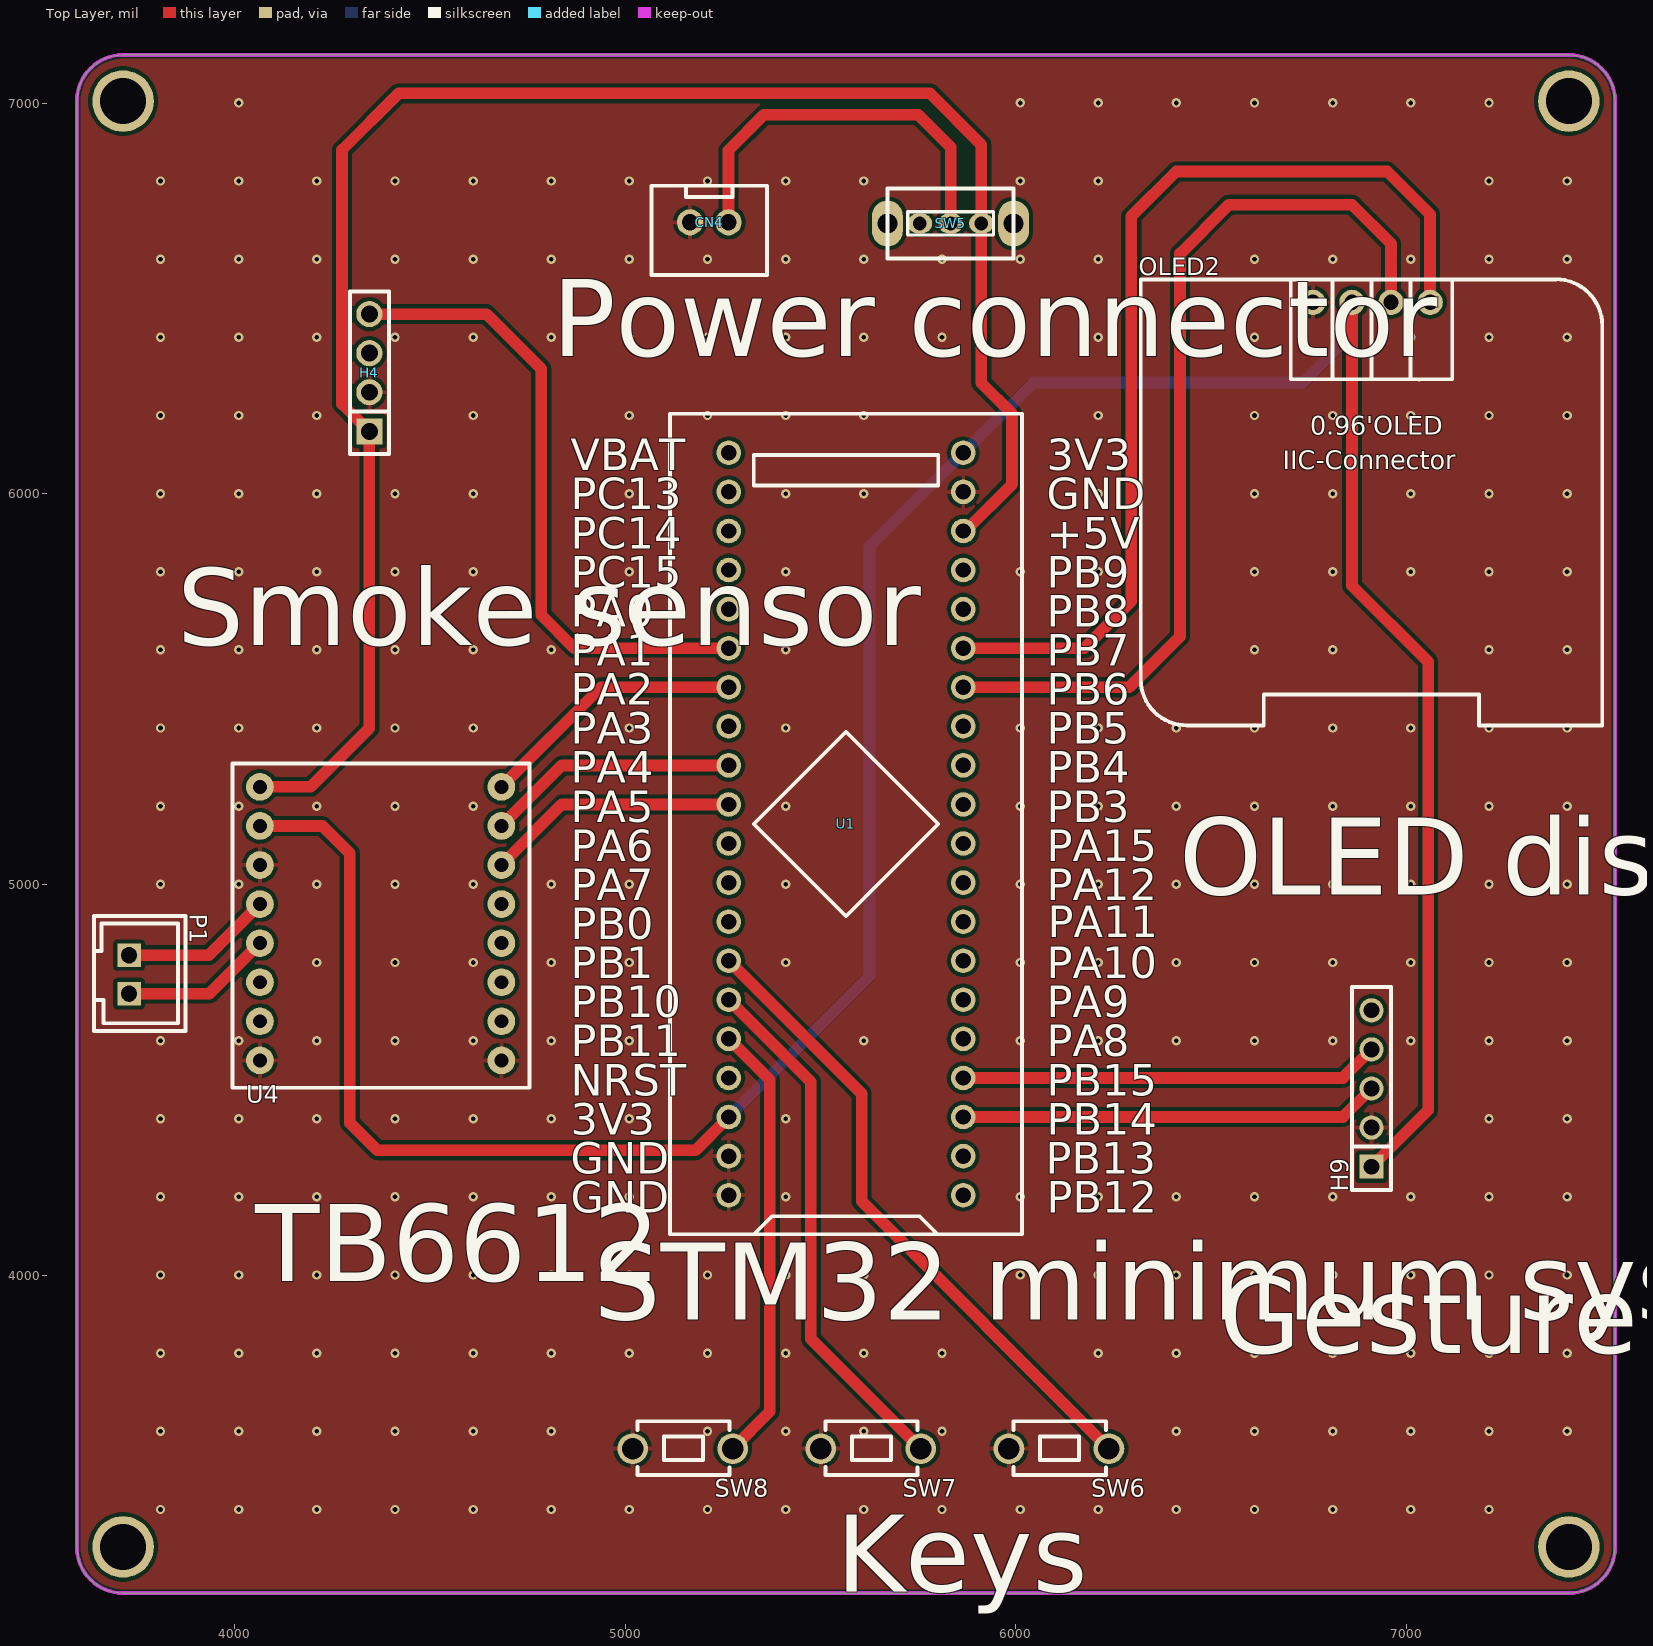
[diagram p0: Top Layer view]
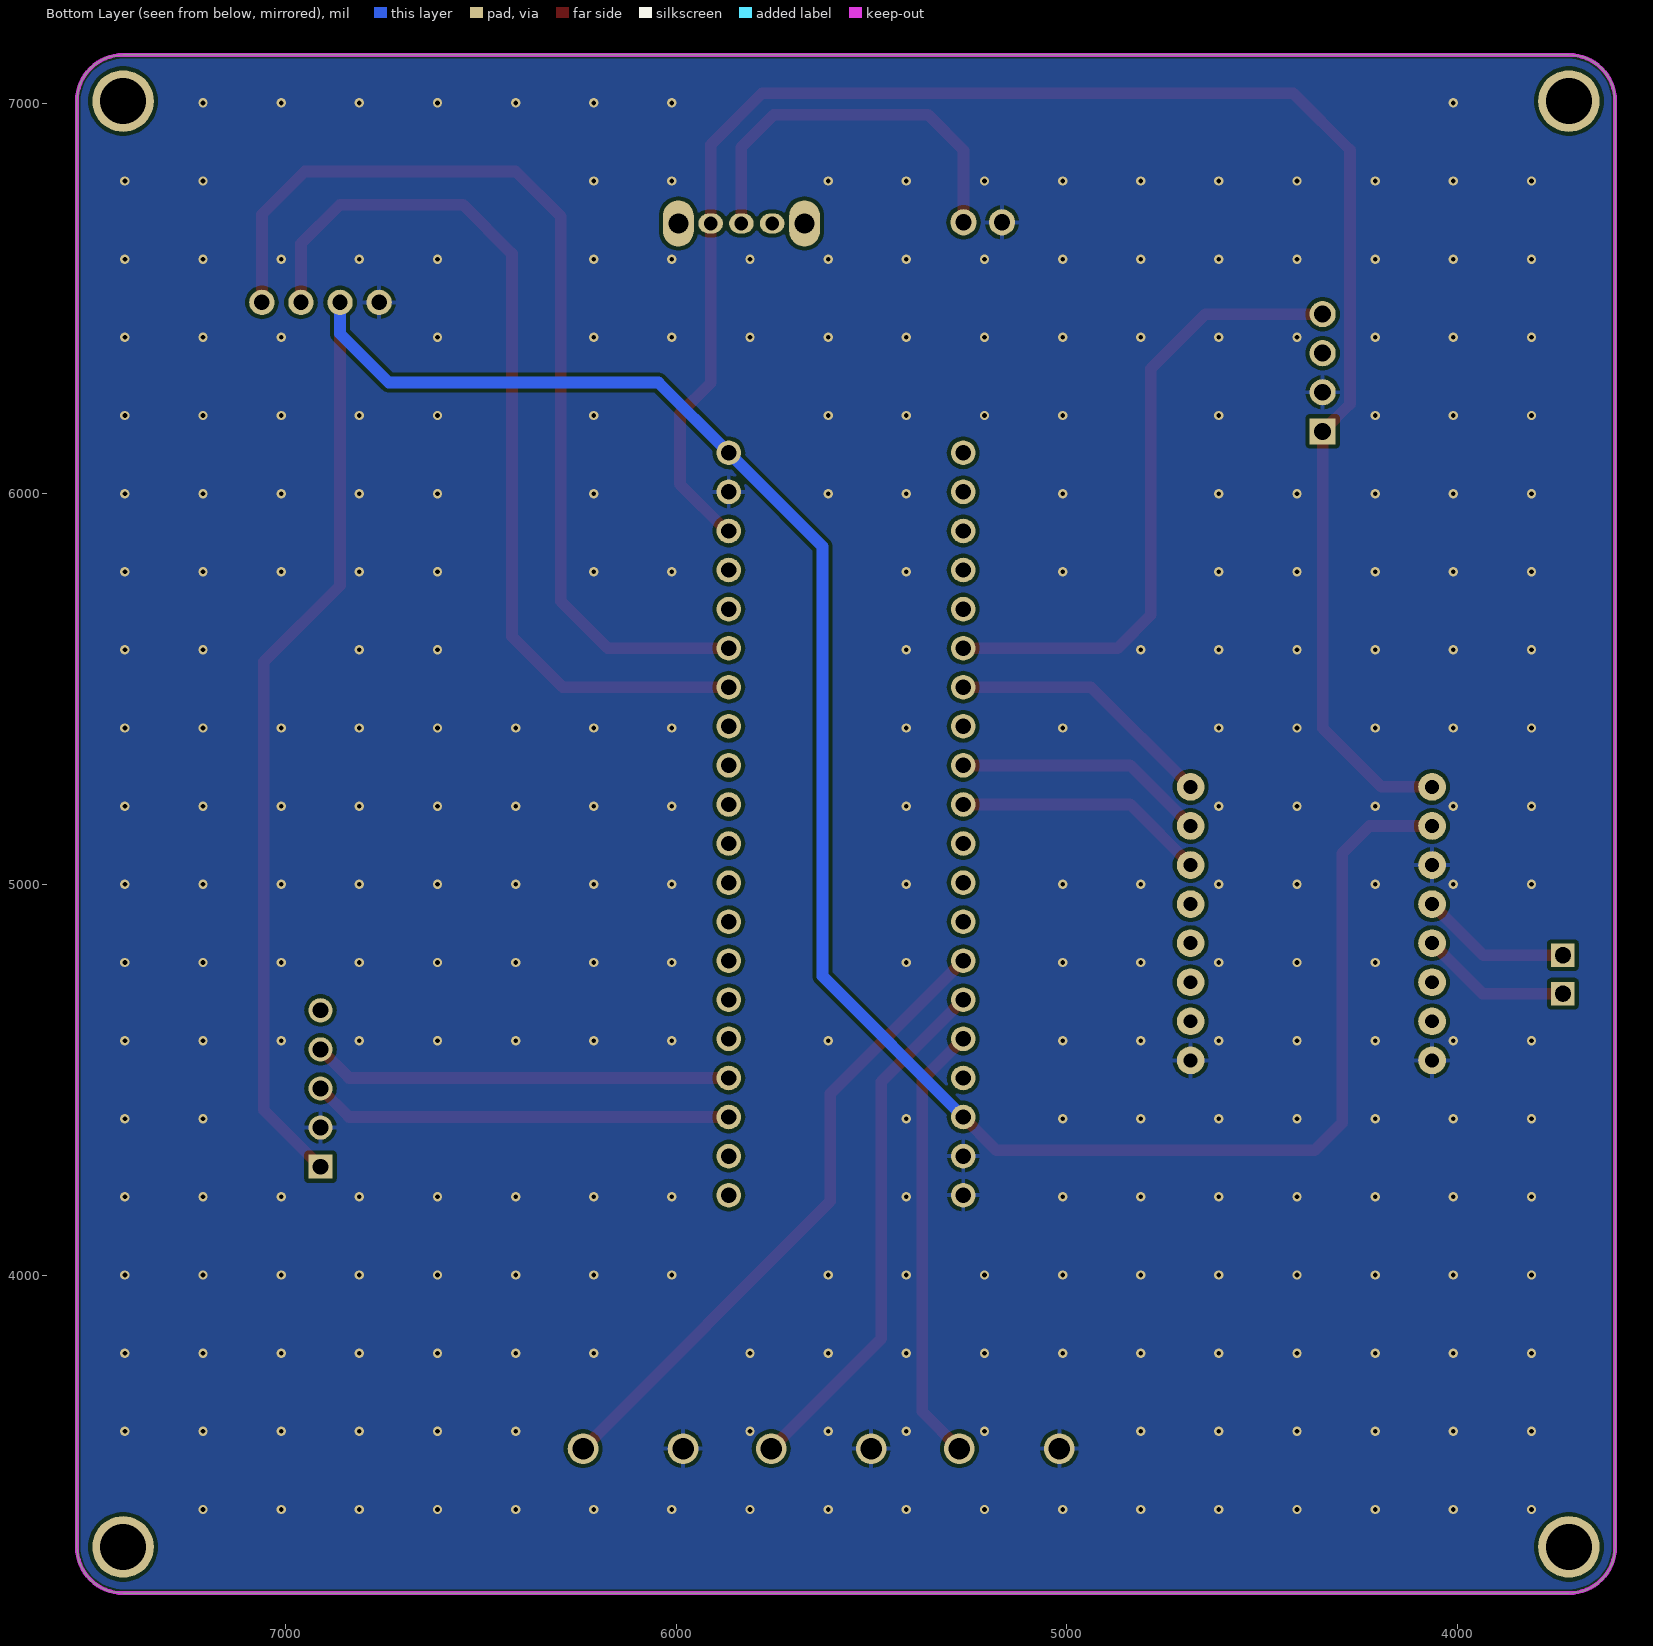
[diagram p1: Bottom Layer view, seen from below]
# Altium PCB MISC89068.pcbdoc
Units mil, origin at the board's own origin, x right, y up, seen from the top; angles counter-clockwise.
Board outline 3937.01 x 3937.01 mil, 2 copper layers (Top Layer, Bottom Layer), stack 62.206 mil thick; 11 components, 40 nets, 88 pads, 281 vias.

## Layer stack, top to bottom
Top Solder Mask Layer: solder mask 0.394, Dk 3.3
Top Layer: signal copper 1.379
Dielectric1: surface 59.449, FR4, Dk 4.5
Bottom Layer: signal copper 1.378
Bottom Solder Mask Layer: solder mask 0.394, Dk 3.3

## Board outline
3714.61,7123.5 ccw(c3714.61,7005.39) 3596.5,7005.39 3596.5,3304.61 ccw(c3714.61,3304.61) 3714.61,3186.5 7415.39,3186.5 ccw(c7415.39,3304.61) 7533.5,3304.61 7533.5,7005.39 ccw(c7415.39,7005.39) 7415.39,7123.5 3714.61,7123.5

## Design rules (kind name [scope] priority, off if disabled: settings)
BoardOutlineClearance copperThickness2oz_1 [All] p2 off: genericclearance=7.99 ignorepadtopadclearanceinfootprint=FALSE except(0: Arc-SplitContinuation Track-SplitContinuation SMDPad-SplitContinuation THPad-SplitContinuation Via-SplitContinuation Fill-SplitContinuation Region-SplitContinuation Poly-SplitContinuation Text-SplitContinuation Hole-SplitContinuation; 5.98: Arc-CutoutEdge Track-CutoutEdge SMDPad-CutoutEdge THPad-CutoutEdge Via-CutoutEdge Text-CutoutEdge; 6.9: Hole-OutlineEdge Hole-CutoutEdge; 10: Poly-OutlineEdge Poly-CutoutEdge; 11.81: Arc-OutlineEdge Track-OutlineEdge SMDPad-OutlineEdge THPad-OutlineEdge Via-OutlineEdge Fill-OutlineEdge Region-OutlineEdge Text-OutlineEdge Fill-CutoutEdge Region-CutoutEdge)
BoardOutlineClearance Plane_innerPlane_1 [All] p4 off: genericclearance=4.02 ignorepadtopadclearanceinfootprint=FALSE except(0: Arc-SplitContinuation Track-SplitContinuation SMDPad-SplitContinuation THPad-SplitContinuation Via-SplitContinuation Fill-SplitContinuation Region-SplitContinuation Poly-SplitContinuation Text-SplitContinuation Hole-SplitContinuation; 5.98: Arc-CutoutEdge Track-CutoutEdge SMDPad-CutoutEdge THPad-CutoutEdge Via-CutoutEdge Text-CutoutEdge; 6.9: Hole-OutlineEdge Hole-CutoutEdge; 10: Poly-OutlineEdge Poly-CutoutEdge; 11.81: Arc-OutlineEdge Track-OutlineEdge SMDPad-OutlineEdge THPad-OutlineEdge Via-OutlineEdge Fill-OutlineEdge Region-OutlineEdge Text-OutlineEdge Fill-CutoutEdge Region-CutoutEdge)
BoardOutlineClearance Copper_copperRegion_1 [All] p6 off: genericclearance=4.02 ignorepadtopadclearanceinfootprint=FALSE except(0: Arc-SplitContinuation Track-SplitContinuation SMDPad-SplitContinuation THPad-SplitContinuation Via-SplitContinuation Fill-SplitContinuation Region-SplitContinuation Poly-SplitContinuation Text-SplitContinuation Hole-SplitContinuation; 5.98: Arc-CutoutEdge Track-CutoutEdge SMDPad-CutoutEdge THPad-CutoutEdge Via-CutoutEdge Text-CutoutEdge; 6.9: Hole-OutlineEdge Hole-CutoutEdge; 10: Poly-OutlineEdge Poly-CutoutEdge; 11.81: Arc-OutlineEdge Track-OutlineEdge SMDPad-OutlineEdge THPad-OutlineEdge Via-OutlineEdge Fill-OutlineEdge Region-OutlineEdge Text-OutlineEdge Fill-CutoutEdge Region-CutoutEdge)
BoardOutlineClearance Copper_copperRegion_copperThickness1oz_1 [All] p8 off: genericclearance=4.02 ignorepadtopadclearanceinfootprint=FALSE except(0: Arc-SplitContinuation Track-SplitContinuation SMDPad-SplitContinuation THPad-SplitContinuation Via-SplitContinuation Fill-SplitContinuation Region-SplitContinuation Poly-SplitContinuation Text-SplitContinuation Hole-SplitContinuation; 5.98: Arc-CutoutEdge Track-CutoutEdge SMDPad-CutoutEdge THPad-CutoutEdge Via-CutoutEdge Text-CutoutEdge; 6.9: Hole-OutlineEdge Hole-CutoutEdge; 10: Poly-OutlineEdge Poly-CutoutEdge; 11.81: Arc-OutlineEdge Track-OutlineEdge SMDPad-OutlineEdge THPad-OutlineEdge Via-OutlineEdge Fill-OutlineEdge Region-OutlineEdge Text-OutlineEdge Fill-CutoutEdge Region-CutoutEdge)
BoardOutlineClearance Copper_copperRegion_Copper_copperRegion_1 [All] p10 off: genericclearance=4.02 ignorepadtopadclearanceinfootprint=FALSE except(0: Arc-SplitContinuation Track-SplitContinuation SMDPad-SplitContinuation THPad-SplitContinuation Via-SplitContinuation Fill-SplitContinuation Region-SplitContinuation Poly-SplitContinuation Text-SplitContinuation Hole-SplitContinuation; 5.98: Arc-CutoutEdge Track-CutoutEdge SMDPad-CutoutEdge THPad-CutoutEdge Via-CutoutEdge Text-CutoutEdge; 6.9: Hole-OutlineEdge Hole-CutoutEdge; 10: Poly-OutlineEdge Poly-CutoutEdge; 11.81: Arc-OutlineEdge Track-OutlineEdge SMDPad-OutlineEdge THPad-OutlineEdge Via-OutlineEdge Fill-OutlineEdge Region-OutlineEdge Text-OutlineEdge Fill-CutoutEdge Region-CutoutEdge)
BoardOutlineClearance copperThickness1oz_1 [All] p12: genericclearance=4.02 ignorepadtopadclearanceinfootprint=FALSE except(0: Arc-SplitContinuation Track-SplitContinuation SMDPad-SplitContinuation THPad-SplitContinuation Via-SplitContinuation Fill-SplitContinuation Region-SplitContinuation Poly-SplitContinuation Text-SplitContinuation Hole-SplitContinuation; 5.98: Arc-CutoutEdge Track-CutoutEdge SMDPad-CutoutEdge THPad-CutoutEdge Via-CutoutEdge Text-CutoutEdge; 6.9: Hole-OutlineEdge Hole-CutoutEdge; 10: Poly-OutlineEdge Poly-CutoutEdge; 11.81: Arc-OutlineEdge Track-OutlineEdge SMDPad-OutlineEdge THPad-OutlineEdge Via-OutlineEdge Fill-OutlineEdge Region-OutlineEdge Text-OutlineEdge Fill-CutoutEdge Region-CutoutEdge)
Clearance copperThickness2oz [All] p1 off: gap=7.99 ignorepadtopadclearanceinfootprint=FALSE except(5.98: SMDPad-Track SMDPad-SMDPad THPad-Track SMDPad-THPad THPad-THPad Track-Via SMDPad-Via THPad-Via Via-Via Fill-SMDPad Region-SMDPad Fill-THPad Region-THPad Fill-Via Region-Via Fill-Fill Fill-Region Region-Region Arc-Track Arc-SMDPad Arc-THPad Arc-Via Fill-Arc Region-Arc Arc-Arc Text-Track SMDPad-Text Text-THPad Text-Via Fill-Text Region-Text Arc-Text Text-Text; 6.9: Hole-Track Hole-SMDPad Hole-THPad Hole-Via Fill-Hole Region-Hole Hole-Arc Hole-Text; 10: Poly-Track Poly-SMDPad Poly-THPad Poly-Via Poly-Fill Poly-Region Poly-Poly Poly-Arc Poly-Text Poly-Hole; 11.81: Fill-Track Region-Track)
Clearance Plane_innerPlane [All] p3 off: gap=4.02 ignorepadtopadclearanceinfootprint=FALSE except(5.98: SMDPad-Track SMDPad-SMDPad THPad-Track SMDPad-THPad THPad-THPad Track-Via SMDPad-Via THPad-Via Via-Via Fill-SMDPad Region-SMDPad Fill-THPad Region-THPad Fill-Via Region-Via Fill-Fill Fill-Region Region-Region Arc-Track Arc-SMDPad Arc-THPad Arc-Via Fill-Arc Region-Arc Arc-Arc Text-Track SMDPad-Text Text-THPad Text-Via Fill-Text Region-Text Arc-Text Text-Text; 6.9: Hole-Track Hole-SMDPad Hole-THPad Hole-Via Fill-Hole Region-Hole Hole-Arc Hole-Text; 10: Poly-Track Poly-SMDPad Poly-THPad Poly-Via Poly-Fill Poly-Region Poly-Poly Poly-Arc Poly-Text Poly-Hole; 11.81: Fill-Track Region-Track)
Clearance Copper_copperRegion [All] p5 off: gap=4.02 ignorepadtopadclearanceinfootprint=FALSE except(5.98: SMDPad-Track SMDPad-SMDPad THPad-Track SMDPad-THPad THPad-THPad Track-Via SMDPad-Via THPad-Via Via-Via Fill-SMDPad Region-SMDPad Fill-THPad Region-THPad Fill-Via Region-Via Fill-Fill Fill-Region Region-Region Arc-Track Arc-SMDPad Arc-THPad Arc-Via Fill-Arc Region-Arc Arc-Arc Text-Track SMDPad-Text Text-THPad Text-Via Fill-Text Region-Text Arc-Text Text-Text; 6.9: Hole-Track Hole-SMDPad Hole-THPad Hole-Via Fill-Hole Region-Hole Hole-Arc Hole-Text; 10: Poly-Track Poly-SMDPad Poly-THPad Poly-Via Poly-Fill Poly-Region Poly-Poly Poly-Arc Poly-Text Poly-Hole; 11.81: Fill-Track Region-Track)
Clearance Copper_copperRegion_copperThickness1oz [All] p7 off: gap=4.02 ignorepadtopadclearanceinfootprint=FALSE except(5.98: SMDPad-Track SMDPad-SMDPad THPad-Track SMDPad-THPad THPad-THPad Track-Via SMDPad-Via THPad-Via Via-Via Fill-SMDPad Region-SMDPad Fill-THPad Region-THPad Fill-Via Region-Via Fill-Fill Fill-Region Region-Region Arc-Track Arc-SMDPad Arc-THPad Arc-Via Fill-Arc Region-Arc Arc-Arc Text-Track SMDPad-Text Text-THPad Text-Via Fill-Text Region-Text Arc-Text Text-Text; 6.9: Hole-Track Hole-SMDPad Hole-THPad Hole-Via Fill-Hole Region-Hole Hole-Arc Hole-Text; 10: Poly-Track Poly-SMDPad Poly-THPad Poly-Via Poly-Fill Poly-Region Poly-Poly Poly-Arc Poly-Text Poly-Hole; 11.81: Fill-Track Region-Track)
Clearance Copper_copperRegion_Copper_copperRegion [All] p9 off: gap=4.02 ignorepadtopadclearanceinfootprint=FALSE except(5.98: SMDPad-Track SMDPad-SMDPad THPad-Track SMDPad-THPad THPad-THPad Track-Via SMDPad-Via THPad-Via Via-Via Fill-SMDPad Region-SMDPad Fill-THPad Region-THPad Fill-Via Region-Via Fill-Fill Fill-Region Region-Region Arc-Track Arc-SMDPad Arc-THPad Arc-Via Fill-Arc Region-Arc Arc-Arc Text-Track SMDPad-Text Text-THPad Text-Via Fill-Text Region-Text Arc-Text Text-Text; 6.9: Hole-Track Hole-SMDPad Hole-THPad Hole-Via Fill-Hole Region-Hole Hole-Arc Hole-Text; 10: Poly-Track Poly-SMDPad Poly-THPad Poly-Via Poly-Fill Poly-Region Poly-Poly Poly-Arc Poly-Text Poly-Hole; 11.81: Fill-Track Region-Track)
Clearance copperThickness1oz [All] p11: gap=4.02 ignorepadtopadclearanceinfootprint=FALSE except(5.98: SMDPad-Track SMDPad-SMDPad THPad-Track SMDPad-THPad THPad-THPad Track-Via SMDPad-Via THPad-Via Via-Via Fill-SMDPad Region-SMDPad Fill-THPad Region-THPad Fill-Via Region-Via Fill-Fill Fill-Region Region-Region Arc-Track Arc-SMDPad Arc-THPad Arc-Via Fill-Arc Region-Arc Arc-Arc Text-Track SMDPad-Text Text-THPad Text-Via Fill-Text Region-Text Arc-Text Text-Text; 6.9: Hole-Track Hole-SMDPad Hole-THPad Hole-Via Fill-Hole Region-Hole Hole-Arc Hole-Text; 10: Poly-Track Poly-SMDPad Poly-THPad Poly-Via Poly-Fill Poly-Region Poly-Poly Poly-Arc Poly-Text Poly-Hole; 11.81: Fill-Track Region-Track)
DiffPairsRouting differentialPair [All] p1: maxlimit=6 minlimit=6 mostfreqgap=6 toplayer_minwidth=5 toplayer_prefwidth=10 toplayer_maxwidth=100 toplayer_mingap=6 toplayer_prefgap=6 toplayer_maxgap=6 bottomlayer_minwidth=5 bottomlayer_prefwidth=10 bottomlayer_maxwidth=100 bottomlayer_mingap=6 bottomlayer_prefgap=6 bottomlayer_maxgap=6 maxuncoupledlength=10
HoleToHoleClearance otherClearance [All] p1: gap=11.81 allowstackedmicrovias=TRUE
Length netLength [All] p1: minlimit=0 maxlimit=0
PasteMaskExpansion pasteMaskExpansion [All] p1: expansion=0
PlaneConnect innerPlane [All] p1: planeconnectstyle=Relief reliefexpansion=20 reliefentries=4 reliefconductorwidth=10 reliefairgap=10
PolygonConnect copperRegion_copperThickness1oz [All] p1 off: connectstyle=Relief reliefconductorwidth=10 reliefentries=4 polygonreliefangle="90 Angle" airgapwidth=10 via.connectstyle=Relief via.reliefconductorwidth=10 via.reliefentries=4 via.polygonreliefangle="90 Angle" via.airgapwidth=10
PolygonConnect copperRegion_Copper_copperRegion [All] p2 off: connectstyle=Relief reliefconductorwidth=10 reliefentries=4 polygonreliefangle="90 Angle" airgapwidth=10 via.connectstyle=Relief via.reliefconductorwidth=10 via.reliefentries=4 via.polygonreliefangle="90 Angle" via.airgapwidth=10
PolygonConnect copperRegion [All] p3: connectstyle=Relief reliefconductorwidth=10 reliefentries=4 polygonreliefangle="90 Angle" airgapwidth=10 via.connectstyle=Relief via.reliefconductorwidth=10 via.reliefentries=4 via.polygonreliefangle="90 Angle" via.airgapwidth=10
RoutingVias viaSize [All] p1: holewidth=12.01 width=24.02 viastyle="Through Hole" minholewidth=11.81 minwidth=19.68 maxholewidth=248.03 maxwidth=393.7
SolderMaskExpansion solderMaskExpansion [IsVia] p1: expansion=-1000 istentingtop=TRUE
SolderMaskExpansion solderMaskExpansion [All] p2: expansion=2 istentingtop=FALSE
Width copperThickness2oz_2 [All] p1 off: maxlimit=100 minlimit=8 preferedwidth=10
Width copperThickness1oz_2 [All] p2: maxlimit=100 minlimit=5 preferedwidth=10

## Components (designator, comment, footprint, x,y, rotation, side; value= is the part's Value field where it differs from the comment)
CN4 "XH2.54*2P_through-hole" CONN-TH_2P-P2.50-XH2.54-2P 5215,6695 r0 top
H4 "" HDR-TH_4P-P2.54-V-F 4345,6310 r90 top
H9 "" HDR-TH_5P-P2.54-V-F 6910,4478.07 r90 top
OLED2 "" 0.96OLED_4P 6910,6490 r0 top
P1 "XH2.54 through-hole socket-2P" CONN-TH_XH2.54-2P 3730,4770 r270 top
SW5 "" 拨动开关 5837.9,6692.05 r180 top
SW6 "" Key_TH_3.5x6x4.3 6116.42,3556.3 r180 top
SW7 "" Key_TH_3.5x6x4.3 5634.97,3556.3 r180 top
SW8 "" Key_TH_3.5x6x4.3 5153.52,3556.3 r180 top
U1 "STM32F103C8T6-Card" CONN-TH_L53.3-W22.9_STM32F103C8T6-CARD 5565,5155 r90 top
U4 "" tb6612 4065,5250 r0 top

## Footprints (in the part's own frame and the unit in brackets; to place one, negate y for a bottom-side part, rotate by r counter-clockwise, add the part's x,y. Pads: shape width x height; smd on the part's side, far side on the other; paste and mask are expansions set on the pad)
0.96OLED_4P [mm]
  round 1.65 hole 1 copper offset 0,0: 1(-3.81,-0.001) 2(-1.27,0.002) 3(1.27,0.002) 4(3.81,0.002)
  silkscreen extent -15,-27.5 15,1.5
CONN-TH_2P-P2.50-XH2.54-2P [mm]
  round 1.7 hole 1.05 paste+0 mask+0.05: 1(1.25,0) 2(-1.25,0)
  silkscreen extent -3.75,-3.42 3.75,2.37
CONN-TH_L53.3-W22.9_STM32F103C8T6-CARD [mm]
  round 1.6 hole 1: 1(-24.13,-7.62) 2(-21.59,-7.62) 3(-19.05,-7.62) 4(-16.51,-7.62) 5(-13.97,-7.62) 6(-11.43,-7.62) 7(-8.89,-7.62) 8(-6.35,-7.62) 9(-3.81,-7.62) 10(-1.27,-7.62) 11(1.27,-7.62) 12(3.81,-7.62) 13(6.35,-7.62) 14(8.89,-7.62) 15(11.43,-7.62) 16(13.97,-7.62) 17(16.51,-7.62) 18(19.05,-7.62) 19(21.59,-7.62) 20(24.13,-7.62) 21(24.13,7.62) 22(21.59,7.62) 23(19.05,7.62) 24(16.51,7.62) 25(13.97,7.62) 26(11.43,7.62) 27(8.89,7.62) 28(6.35,7.62) 29(3.81,7.62) 30(1.27,7.62) 31(-1.27,7.62) 32(-3.81,7.62) 33(-6.35,7.62) 34(-8.89,7.62) 35(-11.43,7.62) 36(-13.97,7.62) 37(-16.51,7.62) 38(-19.05,7.62) 39(-21.59,7.62) 40(-24.13,7.62)
  silkscreen extent -26.67,-11.43 26.67,11.43
CONN-TH_XH2.54-2P [mil]
  rect 60x60 hole 39.37 slot 41.34 at 0 deg paste+0 mask+1.97: 1(-49.22,0) 2(49.21,0)
  silkscreen extent -150,-90 145,145
HDR-TH_4P-P2.54-V-F [mm]
  rect 1.7x1.7 hole 1.1: 1(-3.81,0)
  round 1.7 hole 1.1: 2(-1.27,0) 3(1.27,0) 4(3.81,0)
  silkscreen extent -5.29,-1.27 5.29,1.27
HDR-TH_5P-P2.54-V-F [mil]
  rect 62x62 hole 40.16: 1(-200,0)
  round 62 hole 40.16: 2(-100,0) 3(0,0) 4(100,0) 5(200,0)
  silkscreen extent -260,-50 260,50
Key_TH_3.5x6x4.3 [mil]
  round 78.7 hole 55.1 paste+0 mask+2: A(-121.44,0) B(134.46,0)
  silkscreen extent -114,-70 123,68
tb6612 [mm]
  round 1.8 hole 0.9: 1(0,0) 2(0,-2.54) 3(0,-5.08) 4(0,-7.62) 5(0,-10.16) 6(0,-12.7) 7(0,-15.24) 8(0,-17.78) 9(15.697,-17.78) 10(15.697,-15.24) 11(15.697,-12.7) 12(15.697,-10.16) 13(15.697,-7.62) 14(15.697,-5.08) 15(15.697,-2.54) 16(15.697,0)
  silkscreen extent -1.78,-19.56 17.53,1.52
拨动开关 [mil]
  oval 63x51.2 hole 35.4 paste+0 mask+2: 1(-73.4,0) 2(5,0) 3(84,0)
  oval 78.7x118.1 hole 51.2 paste+0 mask+2: 4(166.7,0) 5(-156.1,0)
  silkscreen extent -156,-90 167,90

## Free pads (board coordinates)
  round 157.48 hole 118.11: 1(3714.61,7005.39) 1(3714.61,3304.61) 1(7415.39,7005.39) 1(7415.39,3304.61)

## Via types
v1: diameter 24.02, hole 12, Top Layer to Bottom Layer, 281 vias

## Nets (pads, with @x,y where several pads share a name; then routed paths per layer and width w, separated by ;. In a path a pad name is that pad's centre, name@x,y a point inside that pad or via, vN(x,y) a via of type N, cw(c..) or ccw(c..) an arc to the next point about the centre after c; other vN are vias at no path point)
$1N17118: CN4.1 SW5.2 | length 1019.9
  Top Layer w30: CN4.1 5264.22,6879.22 5355,6970 5750,6970 5832.9,6887.1 SW5.2
$1N17257: P1.1 U4.4 | length 389.2
  Top Layer w30: P1.1 3934.22,4819.22 U4.4
$1N17258: P1.2 U4.5 | length 388.5
  Top Layer w30: P1.2 3935.78,4720.78 U4.5
+5V: H4.1 SW5.1 U1.18 U4.1 | length 4677.9
  Top Layer w30: U4.1 4195,5250 4345,5400 H4.1 4275,6230 4275,6880 4420,7025 5780,7025 5911.3,6893.7 SW5.1 5911.3,6283.7 5990,6205 5990,6025 5870,5905 U1.18
GND: CN4.2 H4.2 H9.2 OLED2.1 SW6.B SW7.B SW8.B U1.19 U1.39 U1.40 U4.3 U4.8 U4.9
  other v1: 3810.6,3400.6 4010.6,3400.6 4210.6,3400.6 4410.6,3400.6 4610.6,3400.6 4810.6,3400.6 5010.6,3400.6 5210.6,3400.6 5410.6,3400.6 5610.6,3400.6 5810.6,3400.6 6010.6,3400.6 6210.6,3400.6 6410.6,3400.6 6610.6,3400.6 6810.6,3400.6 7010.6,3400.6 7210.6,3400.6 3810.6,3600.6 4010.6,3600.6 4210.6,3600.6 4410.6,3600.6 4610.6,3600.6 4810.6,3600.6 5210.6,3600.6 5410.6,3600.6 5610.6,3600.6 5810.6,3600.6 6410.6,3600.6 6610.6,3600.6 6810.6,3600.6 7010.6,3600.6 7210.6,3600.6 7410.6,3600.6 3810.6,3800.6 4010.6,3800.6 4210.6,3800.6 4410.6,3800.6 4610.6,3800.6 4810.6,3800.6 5010.6,3800.6 5210.6,3800.6 5410.6,3800.6 5610.6,3800.6 5810.6,3800.6 6210.6,3800.6 6410.6,3800.6 6610.6,3800.6 6810.6,3800.6 7010.6,3800.6 7210.6,3800.6 7410.6,3800.6 3810.6,4000.6 4010.6,4000.6 4210.6,4000.6 4410.6,4000.6 4610.6,4000.6 4810.6,4000.6 5010.6,4000.6 5210.6,4000.6 5410.6,4000.6 5610.6,4000.6 6010.6,4000.6 6210.6,4000.6 6410.6,4000.6 6610.6,4000.6 6810.6,4000.6 7010.6,4000.6 7210.6,4000.6 7410.6,4000.6 3810.6,4200.6 4010.6,4200.6 4210.6,4200.6 4410.6,4200.6 4610.6,4200.6 4810.6,4200.6 5010.6,4200.6 5410.6,4200.6 6010.6,4200.6 6210.6,4200.6 6410.6,4200.6 6610.6,4200.6 6810.6,4200.6 7010.6,4200.6 7210.6,4200.6 7410.6,4200.6 3810.6,4400.6 4010.6,4400.6 4210.6,4400.6 4410.6,4400.6 4610.6,4400.6 4810.6,4400.6 5010.6,4400.6 5410.6,4400.6 7210.6,4400.6 7410.6,4400.6 3810.6,4600.6 4010.6,4600.6 4210.6,4600.6 4410.6,4600.6 4610.6,4600.6 4810.6,4600.6 5010.6,4600.6 5610.6,4600.6 6010.6,4600.6 6210.6,4600.6 6410.6,4600.6 6610.6,4600.6 6810.6,4600.6 7010.6,4600.6 7210.6,4600.6 7410.6,4600.6 4210.6,4800.6 4410.6,4800.6 4610.6,4800.6 4810.6,4800.6 5010.6,4800.6 5410.6,4800.6 6010.6,4800.6 6210.6,4800.6 6410.6,4800.6 6610.6,4800.6 6810.6,4800.6 7010.6,4800.6 7210.6,4800.6 7410.6,4800.6 3810.6,5000.6 4010.6,5000.6 4210.6,5000.6 4410.6,5000.6 4610.6,5000.6 4810.6,5000.6 5010.6,5000.6 5410.6,5000.6 6010.6,5000.6 6210.6,5000.6 6410.6,5000.6 6610.6,5000.6 6810.6,5000.6 7010.6,5000.6 7210.6,5000.6 7410.6,5000.6 3810.6,5200.6 4010.6,5200.6 4210.6,5200.6 4410.6,5200.6 4610.6,5200.6 5410.6,5200.6 6010.6,5200.6 6210.6,5200.6 6410.6,5200.6 6610.6,5200.6 6810.6,5200.6 7010.6,5200.6 7210.6,5200.6 7410.6,5200.6 3810.6,5400.6 4010.6,5400.6 4210.6,5400.6 4410.6,5400.6 4610.6,5400.6 5010.6,5400.6 5410.6,5400.6 6010.6,5400.6 6210.6,5400.6 6410.6,5400.6 6610.6,5400.6 6810.6,5400.6 7010.6,5400.6 7210.6,5400.6 7410.6,5400.6 3810.6,5600.6 4010.6,5600.6 4210.6,5600.6 4410.6,5600.6 4610.6,5600.6 4810.6,5600.6 5410.6,5600.6 6610.6,5600.6 6810.6,5600.6 7210.6,5600.6 7410.6,5600.6 3810.6,5800.6 4010.6,5800.6 4210.6,5800.6 4410.6,5800.6 4610.6,5800.6 5010.6,5800.6 5410.6,5800.6 6010.6,5800.6 6210.6,5800.6 6610.6,5800.6 6810.6,5800.6 7010.6,5800.6 7210.6,5800.6 7410.6,5800.6 3810.6,6000.6 4010.6,6000.6 4210.6,6000.6 4410.6,6000.6 4610.6,6000.6 5010.6,6000.6 5410.6,6000.6 5610.6,6000.6 6210.6,6000.6 6610.6,6000.6 6810.6,6000.6 7010.6,6000.6 7210.6,6000.6 7410.6,6000.6 3810.6,6200.6 4010.6,6200.6 4210.6,6200.6 4610.6,6200.6 5010.6,6200.6 5210.6,6200.6 5410.6,6200.6 5610.6,6200.6 6210.6,6200.6 6610.6,6200.6 6810.6,6200.6 7010.6,6200.6 7210.6,6200.6 7410.6,6200.6 3810.6,6400.6 4010.6,6400.6 4210.6,6400.6 4410.6,6400.6 4610.6,6400.6 4810.6,6400.6 5010.6,6400.6 5210.6,6400.6 5410.6,6400.6 5610.6,6400.6 5810.6,6400.6 6010.6,6400.6 6210.6,6400.6 6610.6,6400.6 7010.6,6400.6 7210.6,6400.6 7410.6,6400.6 3810.6,6600.6 4010.6,6600.6 4210.6,6600.6 4410.6,6600.6 4610.6,6600.6 4810.6,6600.6 5010.6,6600.6 5210.6,6600.6 5410.6,6600.6 5610.6,6600.6 5810.6,6600.6 6010.6,6600.6 6210.6,6600.6 6610.6,6600.6 6810.6,6600.6 7010.6,6600.6 7210.6,6600.6 7410.6,6600.6 3810.6,6800.6 4010.6,6800.6 4210.6,6800.6 4410.6,6800.6 4610.6,6800.6 4810.6,6800.6 5010.6,6800.6 5210.6,6800.6 5410.6,6800.6 5610.6,6800.6 6010.6,6800.6 6210.6,6800.6 7210.6,6800.6 7410.6,6800.6 4010.6,7000.6 6010.6,7000.6 6210.6,7000.6 6410.6,7000.6 6610.6,7000.6 6810.6,7000.6 7010.6,7000.6 7210.6,7000.6
NRST: U1.37
PA0: U1.25
PA1: H4.4 U1.26 | length 1643.2
  Top Layer w30: H4.4 4645,6460 4785,6320 4785,5690 4870,5605 U1.26
PA2: U1.27 U4.16 | length 687.6
  Top Layer w30: U4.16 4938,5505 U1.27
PA3: U1.28
PA4: U1.29 U4.15 | length 646.2
  Top Layer w30: U4.15 4838,5305 U1.29
PA5: U1.30 U4.14 | length 646.2
  Top Layer w30: U4.14 4838,5205 U1.30
PA6: U1.31
PA7: U1.32
PA8: U1.5
PA9: U1.6
PA10: U1.7
PA11: U1.8
PA12: U1.9
PA15: U1.10
PB0: U1.33
PB1: SW6.A U1.34 | length 1651.7
  Top Layer w30: U1.34 5605,4465 5605,4189.16 SW6.A
PB3: U1.11
PB4: U1.12
PB5: U1.13
PB6: OLED2.3 U1.14 | length 2372
  Top Layer w30: U1.14 6290,5505 6420,5635 6420,6615 6545,6740 6860,6740 6960,6640 OLED2.3@6960,6490.05
PB7: OLED2.4 U1.15 | length 2547.9
  Top Layer w30: U1.15 6175,5605 6295,5725 6295,6710 6410,6825 6950,6825 7060,6715 OLED2.4@7060,6490.05
PB8: U1.16
PB9: U1.17
PB10: SW7.A U1.35 | length 1352.3
  Top Layer w30: U1.35 5475,4495 5475,3837.71 SW7.A
PB11: SW8.A U1.36 | length 1131.6
  Top Layer w30: U1.36 5370,4500 5370,3651.34 SW8.A
PB12: U1.1
PB13: U1.2
PB14: H9.3 U1.3 | length 1075.3
  Top Layer w30: U1.3 6836.92,4405 H9.3
PB15: H9.4 U1.4 | length 1075.3
  Top Layer w30: U1.4 6836.92,4505 H9.4
PC13: U1.22
PC14: U1.23
PC15: U1.24
VBAT: U1.21
VCC: H9.1 OLED2.2 U1.20 U1.38 U4.2 | length 7485.9
  Top Layer w30: U4.2 4225,5150 4295,5080 4295,4390 4365,4320 5180,4320 U1.38 ; OLED2.2@6860,6490.05 6860,5765 7055,5570 7055,4423.08 H9.1
  Bottom Layer w30: U1.38 5625,4765 5625,5865 U1.20 6045,6285 6735,6285 6860,6410 OLED2.2@6860,6490.05
pads on no net: H4.3 H9.5 SW5.3 SW5.4 SW5.5 U4.6 U4.7 U4.10 U4.11 U4.12 U4.13

## Polygon pours and split planes (outlines as drawn)
GND on Bottom Layer (solid, remove dead copper, pour order 2): 3525,7245 3525,3080 7700,3080 7700,7245
GND on Top Layer (solid, remove dead copper, pour order 2): 3000,7415 3000,3000 7930,3000 7930,7415

## Keep-outs
Board Outline Layer:
  the board outline again, w10

## Silkscreen, mask and mechanical layers (free items; w line width, h text height)
Top Silkscreen Layer:
  text "Power connector" at 4812.87,6351.57 h196.85
  text "VBAT" at 4860.95,6060 h80
  text "3V3" at 6079.16,6060 h80
  text "PC13" at 4860.95,5960 h80
  text "GND" at 6079.16,5960 h80
  text "PC14" at 4860.95,5860 h80
  text "+5V" at 6079.16,5860 h80
  text "PC15" at 4860.95,5760 h80
  text "PB9" at 6079.16,5760 h80
  text "PA0" at 4860.95,5660 h80
  text "PB8" at 6079.16,5660 h80
  text "Smoke sensor" at 3853.62,5613.07 h196.85
  text "PA1" at 4860.95,5560 h80
  text "PB7" at 6079.16,5560 h80
  text "PA2" at 4860.95,5460 h80
  text "PB6" at 6079.16,5460 h80
  text "PA3" at 4860.95,5360 h80
  text "PB5" at 6079.16,5360 h80
  text "PA4" at 4860.95,5260 h80
  text "PB4" at 6079.16,5260 h80
  text "PA5" at 4860.95,5160 h80
  text "PB3" at 6079.16,5160 h80
  text "PA6" at 4860.95,5060 h80
  text "PA15" at 6079.16,5060 h80
  text "OLED display" at 6418.02,4974.21 h196.85
  text "PA7" at 4860.95,4960 h80
  text "PA12" at 6079.16,4960 h80
  text "PA11" at 6080.95,4865 h80
  text "PB0" at 4860.95,4860 h80
  text "PB1" at 4860.95,4760 h80
  text "PA10" at 6079.16,4760 h80
  text "PB10" at 4860.95,4660 h80
  text "PA9" at 6079.16,4660 h80
  text "PB11" at 4860.95,4560 h80
  text "PA8" at 6079.16,4560 h80
  text "NRST" at 4860.95,4460 h80
  text "PB15" at 6079.16,4460 h80
  text "3V3" at 4860.95,4360 h80
  text "PB14" at 6079.16,4360 h80
  text "GND" at 4860.95,4260 h80
  text "PB13" at 6075.95,4260 h80
  text "GND" at 4860.95,4160 h80
  text "PB12" at 6079.16,4160 h80
  text "TB6612" at 4053.3,3985 h196.85
  text "STM32 minimum system" at 4919.45,3886.57 h196.85
  text "Gesture recognition" at 6520.17,3800 h196.85
  text "Keys" at 5540,3190 h196.85